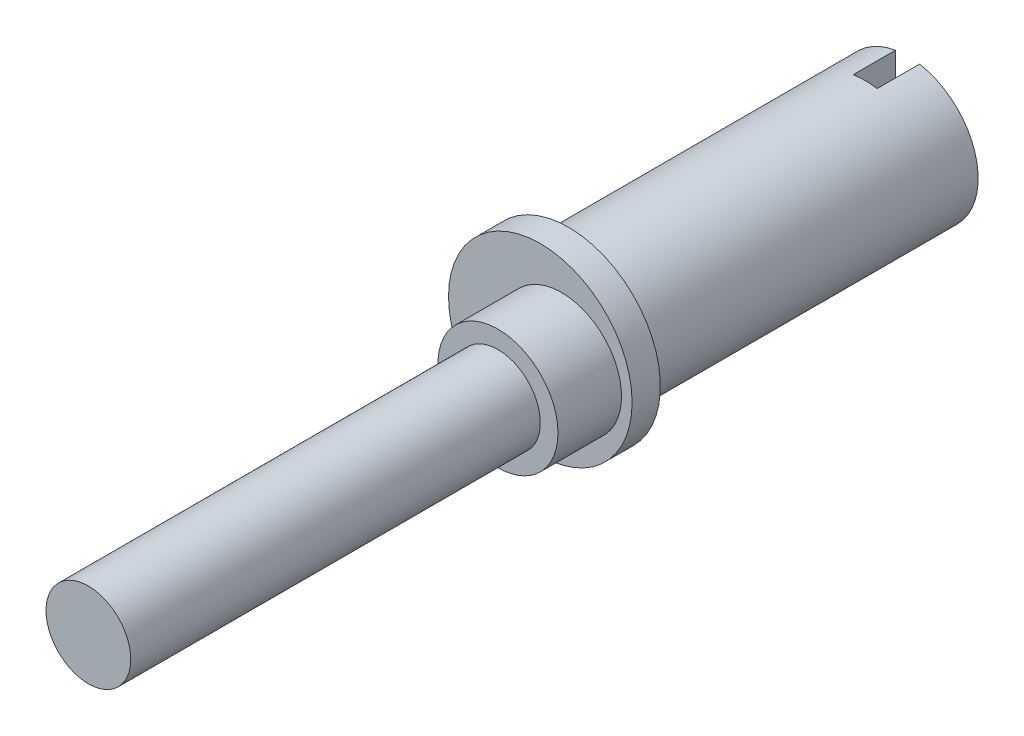
SolidWorks part; units mm, degrees
ref_plane "Front Plane" through (0, 0, 0) normal (0, 0, 1) x (1, 0, 0)
ref_plane "Top Plane" through (0, 0, 0) normal (0, 1, 0) x (1, 0, 0)
ref_plane "Right Plane" through (0, 0, 0) normal (1, 0, 0) x (0, 0, -1)
sketch "Sketch1" plane through (0, 0, 0) normal (0, 0, 1) x (1, 0, 0)
  circle A0 centre (0, 0) radius 5
  dimension "D1" = 10
extrude "Boss-Extrude1" add sketch "Sketch1" along normal blind 25
cosmetic thread "Cosmetic Thread2" parameters "D1"=15, "D2"=8.376
sketch "Sketch2" plane through (0, 0, 25) normal (0, 0, 1) x (1, 0, 0)
  circle A0 centre (0, 0) radius 6.5
  dimension "D1" = 13
extrude "Boss-Extrude2" add sketch "Sketch2" along normal blind 1
sketch "Sketch3" plane through (0, 0, 26) normal (0, 0, 1) x (1, 0, 0)
  line L0 (0, 0) -> (7.1045, 0) construction
  circle A0 centre (1.5, 0) radius 4.25
  dimension "D1" = 8.5
  dimension "D2" = 1.5
extrude "Boss-Extrude3" add sketch "Sketch3" along normal blind 4.5
sketch "Sketch4" plane through (0, 0, 30.5) normal (0, 0, 1) x (1, 0, 0)
  circle A0 centre (1.5, 0) radius 3
  dimension "D1" = 6
extrude "Boss-Extrude4" add sketch "Sketch4" along normal blind 29 contours A0
cosmetic thread "Cosmetic Thread1" parameters "D1"=18, "D2"=4.917
sketch "Sketch6" plane through (0, 0, 0) normal (0, 0, -1) x (-1, 0, 0)
  line L1 (-0.85, 5.9657) -> (0.85, 5.9657)
  line L2 (-0.85, 5.9657) -> (-0.85, -5.9657)
  line L3 (-0.85, -5.9657) -> (0.85, -5.9657)
  line L4 (0.85, 5.9657) -> (0.85, -5.9657)
  line L5 (0, -5.9657) -> (0, 5.9657) construction
  line L6 (-0.85, 0) -> (0.85, 0) construction
  point P0 (0, 0)
  dimension "D1" = 1.7
extrude "Cut-Extrude1" cut sketch "Sketch6" against normal blind 3
sketch "Sketch7" plane through (0, 0, 25) normal (0, 0, -1) x (-1, 0, 0)
  circle A1 centre (0, 0) radius 6.5
  circle A2 centre (0, 0) radius 6.5
  dimension "D1" = 0
extrude "Boss-Extrude5" add sketch "Sketch7" along normal blind 1
